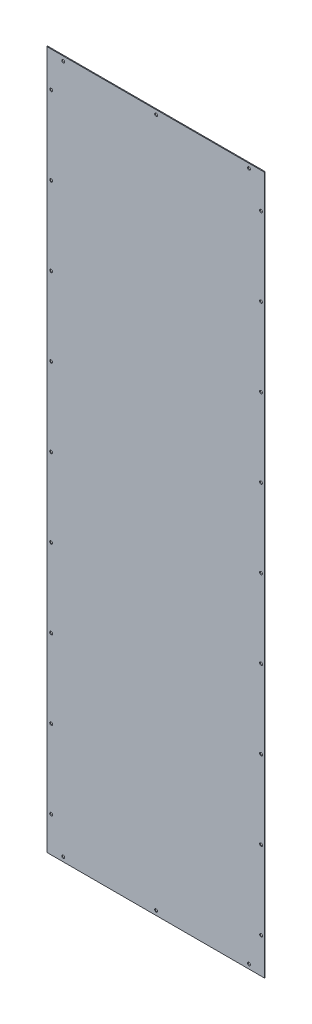
from build123d import *

# Parameters (mm, degrees)
SKETCH_1_W          = 494.5
SKETCH_1_H          = 1578
SKETCH_1_R          = 3.25
EXTRUDE_1_DEPTH     = 2
SKETCH_2_W          = 2.5
SKETCH_2_H          = 2
CUT_EXTRUDE_1_DEPTH = 1598.254069489


with BuildPart() as part:
    # 草图1 → 凸台-拉伸1 (new body)
    with BuildSketch(Plane.XY):
        Rectangle(SKETCH_1_W, SKETCH_1_H)
        with Locations((-237.25, 0)):
            Circle(SKETCH_1_R, mode=Mode.SUBTRACT)
        with Locations((-237.25, -177.25)):
            Circle(SKETCH_1_R, mode=Mode.SUBTRACT)
        with Locations((-237.25, -354.5)):
            Circle(SKETCH_1_R, mode=Mode.SUBTRACT)
        with Locations((-237.25, -531.75)):
            Circle(SKETCH_1_R, mode=Mode.SUBTRACT)
        with Locations((-237.25, -709)):
            Circle(SKETCH_1_R, mode=Mode.SUBTRACT)
        with Locations((0, -779)):
            Circle(SKETCH_1_R, mode=Mode.SUBTRACT)
        with Locations(Location((0, 779, 0), (0, 0, 180))):
            Circle(SKETCH_1_R, mode=Mode.SUBTRACT)
        with Locations(Location((-237.25, 709, 0), (0, 0, 180))):
            Circle(SKETCH_1_R, mode=Mode.SUBTRACT)
        with Locations(Location((-237.25, 531.75, 0), (0, 0, 180))):
            Circle(SKETCH_1_R, mode=Mode.SUBTRACT)
        with Locations(Location((-237.25, 354.5, 0), (0, 0, 180))):
            Circle(SKETCH_1_R, mode=Mode.SUBTRACT)
        with Locations(Location((-237.25, 177.25, 0), (0, 0, 180))):
            Circle(SKETCH_1_R, mode=Mode.SUBTRACT)
        with Locations((237.25, 177.25)):
            Circle(SKETCH_1_R, mode=Mode.SUBTRACT)
        with Locations((237.25, 354.5)):
            Circle(SKETCH_1_R, mode=Mode.SUBTRACT)
        with Locations((237.25, 531.75)):
            Circle(SKETCH_1_R, mode=Mode.SUBTRACT)
        with Locations((237.25, 709)):
            Circle(SKETCH_1_R, mode=Mode.SUBTRACT)
        with Locations(Location((237.25, -709, 0), (0, 0, 180))):
            Circle(SKETCH_1_R, mode=Mode.SUBTRACT)
        with Locations(Location((237.25, -531.75, 0), (0, 0, 180))):
            Circle(SKETCH_1_R, mode=Mode.SUBTRACT)
        with Locations(Location((237.25, -354.5, 0), (0, 0, 180))):
            Circle(SKETCH_1_R, mode=Mode.SUBTRACT)
        with Locations(Location((237.25, -177.25, 0), (0, 0, 180))):
            Circle(SKETCH_1_R, mode=Mode.SUBTRACT)
        with Locations(Location((237.25, 0, 0), (0, 0, 180))):
            Circle(SKETCH_1_R, mode=Mode.SUBTRACT)
        with Locations((-210, 779)):
            Circle(SKETCH_1_R, mode=Mode.SUBTRACT)
        with Locations((210, 779)):
            Circle(SKETCH_1_R, mode=Mode.SUBTRACT)
        with Locations(Location((210, -779, 0), (0, 0, 180))):
            Circle(SKETCH_1_R, mode=Mode.SUBTRACT)
        with Locations(Location((-210, -779, 0), (0, 0, 180))):
            Circle(SKETCH_1_R, mode=Mode.SUBTRACT)
    extrude(amount=EXTRUDE_1_DEPTH)

    # 草图2 → 切除-拉伸1 (cut, through all)
    with BuildSketch(Plane.XZ.offset(789)):
        with Locations((246, 1)):
            Rectangle(SKETCH_2_W, SKETCH_2_H)
    extrude(amount=-CUT_EXTRUDE_1_DEPTH, mode=Mode.SUBTRACT)


solid = part.part
